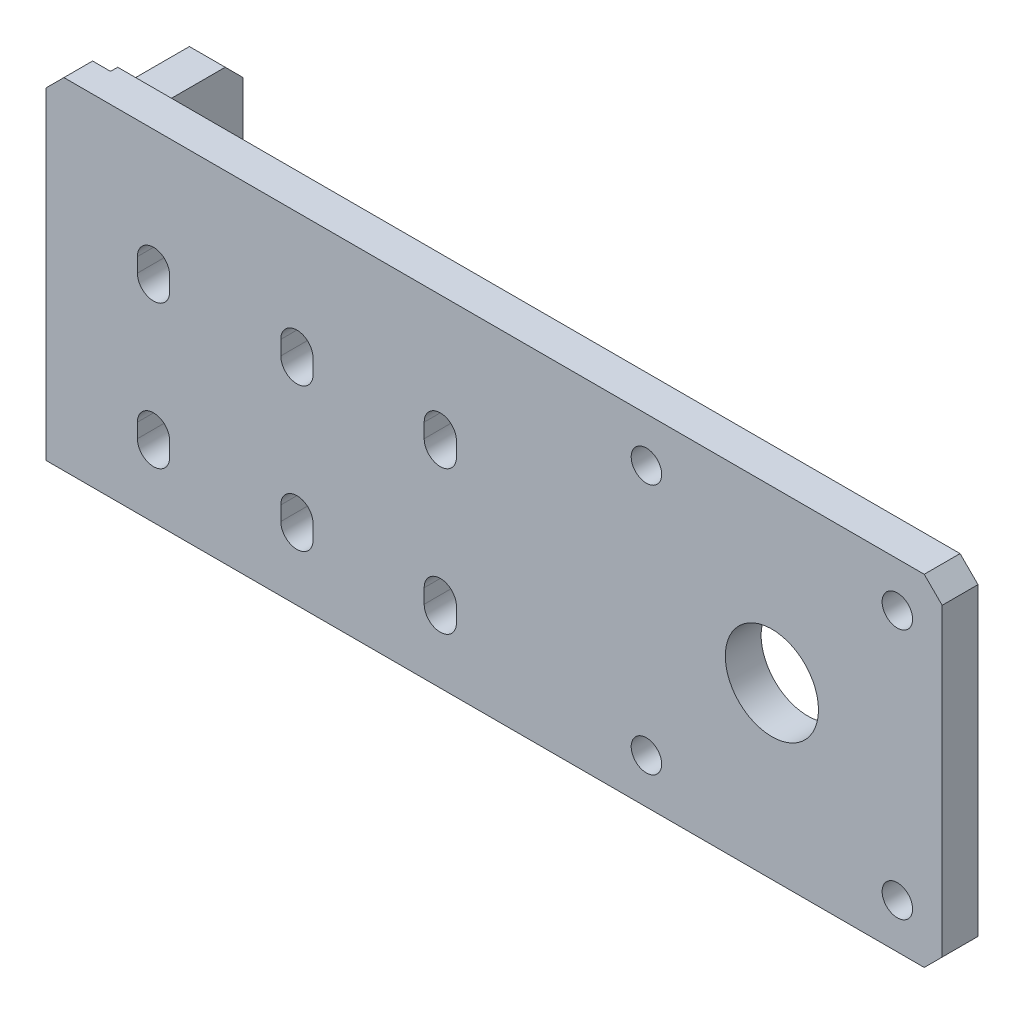
SolidWorks part; units mm, degrees
material "AISI 1045 钢，冷拔"
ref_plane "前视基准面" through (0, 0, 0) normal (0, 0, 1) x (1, 0, 0)
ref_plane "上视基准面" through (0, 0, 0) normal (0, 1, 0) x (1, 0, 0)
ref_plane "右视基准面" through (0, 0, 0) normal (1, 0, 0) x (0, 0, -1)
sketch "草图1" plane through (0, 0, 0) normal (0, 0, 1) x (1, 0, 0)
  line L1 (-125, 47.5) -> (125, 47.5)
  line L2 (-125, 47.5) -> (-125, -47.5)
  line L3 (-125, -47.5) -> (125, -47.5)
  line L4 (125, 47.5) -> (125, -47.5)
  line L5 (-125, 47.5) -> (125, -47.5) construction
  line L6 (-125, -47.5) -> (125, 47.5) construction
  point P0 (0, 0)
  dimension "D1" = 95
  dimension "D2" = 250
extrude "凸台-拉伸1" add sketch "草图1" along normal blind 10
sketch "草图3" plane through (0, 0, 10) normal (0, 0, 1) x (1, 0, 0)
  line L0 (-55, 17.5058) -> (-55, -69.5405) construction
  line L1 (125, -47.5) -> (125, 47.5) construction
  line L2 (-22.9727, -29.5) -> (-57.0867, -29.5) construction
  line L3 (-125, -47.5) -> (125, -47.5) construction
  line L4 (-55, -29.5) -> (-55, -25.5) construction
  line L5 (-59.5, -29.5) -> (-59.5, -25.5)
  line L6 (-50.5, -29.5) -> (-50.5, -25.5)
  arc A0 (-59.5, -29.5) -> (-50.5, -29.5) centre (-55, -29.5) ccw
  arc A1 (-50.5, -25.5) -> (-59.5, -25.5) centre (-55, -25.5) ccw
  point P10 (-55, -27.5)
  dimension "D4" = 4.5
  dimension "D1" = 180
  dimension "D2" = 18
  dimension "D3" = 4
extrude "切除-拉伸2" cut sketch "草图3" against normal through all
pattern_linear "阵列(线性)1" count 2 spacing 40 along (1, 0, 0) count 2 spacing 40 along (0, 1, 0) of "切除-拉伸2"
pattern_linear "阵列(线性)2" count 2 spacing 40 along (-1, 0, 0) count 2 spacing 40 along (0, 1, 0) of "切除-拉伸2"
sketch "草图10" plane through (0, 0, 10) normal (0, 0, 1) x (1, 0, 0)
  line L0 (24.75, 0) -> (-24.75, 0) construction
  line L1 (42.5, 35) -> (112.5, 35) construction
  line L2 (42.5, 35) -> (42.5, -35) construction
  line L3 (42.5, -35) -> (112.5, -35) construction
  line L4 (112.5, 35) -> (112.5, -35) construction
  line L5 (42.5, 35) -> (112.5, -35) construction
  line L6 (42.5, -35) -> (112.5, 35) construction
  line L7 (125, -47.5) -> (125, 47.5) construction
  point P0 (77.5, 0)
  dimension "D1" = 70
  dimension "D2" = 70
  dimension "D3" = 47.5
hole_wizard "M10 螺纹孔3" positions "3D草图3" profile "草图11" tap size "M10" standard "GB"
sketch3d "3D草图3"
  point P0 (42.5, 35, 10)
  point P3 (112.5, 35, 10)
  point P6 (112.5, -35, 10)
  point P9 (42.5, -35, 10)
sketch "草图11" plane through (42.5, 35, 10) normal (1, 0, 0) x (0, -1, 0)
  line L0 (0, 0) -> (0, 27.0537)
  line L1 (0, 27.0537) -> (4.25, 24.5)
  line L2 (4.25, 24.5) -> (4.25, 0)
  line L5 (4.25, 0) -> (0, 0)
  line L10 (0, 27.0537) -> (-4.25, 24.5) construction
  line L11 (0, -6.35) -> (0, 107.95) construction
  dimension "螺纹孔钻头直径" = 8.5
  dimension "螺纹孔钻头深度" = 24.5
  dimension "导头角度" = 118
cosmetic thread "孔螺蚊线9"
cosmetic thread "孔螺蚊线10"
cosmetic thread "孔螺蚊线11"
cosmetic thread "孔螺蚊线12"
sketch "草图12" plane through (0, 0, 10) normal (0, 0, 1) x (1, 0, 0)
  line L0 (42.5, 35) -> (112.5, -35) construction
  circle A0 centre (77.5, 0) radius 13
  dimension "D1" = 26
extrude "切除-拉伸5" cut sketch "草图12" against normal through all
sketch "草图13" plane through (0, 0, 0) normal (0, 0, -1) x (-1, 0, 0)
  line L0 (-45, -20) -> (-110, -20) construction
  line L1 (-110, -20) -> (-110, 20) construction
  line L2 (-110, 20) -> (-45, 20) construction
hole_wizard "M6 螺纹孔1" positions "3D草图4" profile "草图14" tap size "M6" standard "GB"
sketch3d "3D草图4"
  point P0 (45, -20, 0)
  point P3 (110, -20, 0)
  point P6 (110, 20, 0)
  point P9 (45, 20, 0)
sketch "草图14" plane through (45, -20, 0) normal (1, 0, 0) x (0, 1, 0)
  line L0 (0, 0) -> (0, 10)
  line L1 (0, 10) -> (2.5, 10)
  line L2 (2.5, 10) -> (2.5, 0)
  line L5 (2.5, 0) -> (0, 0)
  line L11 (0, -6.35) -> (0, 107.95) construction
  dimension "通孔螺纹孔钻头直径" = 5
  dimension "通孔螺纹孔钻头深度" = 10
cosmetic thread "孔螺蚊线17" [suppressed]
cosmetic thread "孔螺蚊线18" [suppressed]
cosmetic thread "孔螺蚊线19" [suppressed]
cosmetic thread "孔螺蚊线20" [suppressed]
sketch "草图15" plane through (-125, 0, 0) normal (-1, 0, 0) x (0, 0, 1)
  line L0 (5, -37.5) -> (5, -17.5) construction
  line L1 (5, -17.5) -> (5, 2.5) construction
  line L2 (5, 2.5) -> (5, 22.5) construction
hole_wizard "M6 螺纹孔2" positions "3D草图5" profile "草图16" tap size "M6" standard "GB"
sketch3d "3D草图5"
  point P0 (-125, -37.5, 5)
  point P3 (-125, -17.5, 5)
  point P6 (-125, 2.5, 5)
  point P9 (-125, 22.5, 5)
sketch "草图16" plane through (-125, -37.5, 5) normal (0, 1, 0) x (0, 0, 1)
  line L0 (0, 0) -> (0, 16.5022)
  line L1 (0, 16.5022) -> (2.5, 15)
  line L2 (2.5, 15) -> (2.5, 0)
  line L5 (2.5, 0) -> (0, 0)
  line L10 (0, 16.5022) -> (-2.5, 15) construction
  line L11 (0, -6.35) -> (0, 107.95) construction
  dimension "螺纹孔钻头直径" = 5
  dimension "螺纹孔钻头深度" = 15
  dimension "导头角度" = 118
cosmetic thread "孔螺蚊线21" [suppressed]
cosmetic thread "孔螺蚊线22" [suppressed]
cosmetic thread "孔螺蚊线23" [suppressed]
cosmetic thread "孔螺蚊线24" [suppressed]
sketch "草图18" plane through (0, -47.5, 0) normal (0, -1, 0) x (1, 0, 0)
  line L0 (12, 5) -> (47, 5) construction
  line L1 (47, 5) -> (82, 5) construction
  line L2 (82, 5) -> (117, 5) construction
  point P4 (64.5, 5)
hole_wizard "M4 螺纹孔1" positions "3D草图6" profile "草图19" tap size "M4" standard "GB"
sketch3d "3D草图6"
  point P0 (117, -47.5, 5)
  point P9 (12, -47.5, 5)
  point P12 (64.5, -47.5, 5)
sketch "草图19" plane through (117, -47.5, 5) normal (1, 0, 0) x (0, 0, -1)
  line L0 (0, 0) -> (0, 11.0914)
  line L1 (0, 11.0914) -> (1.65, 10.1)
  line L2 (1.65, 10.1) -> (1.65, 0)
  line L5 (1.65, 0) -> (0, 0)
  line L10 (0, 11.0914) -> (-1.65, 10.1) construction
  line L11 (0, -6.35) -> (0, 107.95) construction
  dimension "螺纹孔钻头直径" = 3.3
  dimension "螺纹孔钻头深度" = 10.1
  dimension "导头角度" = 118
cosmetic thread "孔螺蚊线25"
cosmetic thread "孔螺蚊线26"
cosmetic thread "孔螺蚊线28"
sketch "草图22" plane through (0, 0, 0) normal (0, 0, -1) x (-1, 0, 0)
  line L0 (125, -47.5) -> (-125, -47.5) construction
  line L1 (125, 47.5) -> (115, 47.5)
  line L2 (125, 47.5) -> (125, -47.5)
  line L3 (125, -47.5) -> (115, -47.5)
  line L4 (115, 47.5) -> (115, -47.5)
  dimension "D1" = 10
extrude "切除-拉伸6" cut sketch "草图22" against normal blind 2
sketch "草图21" plane through (0, 0, 2) normal (0, 0, -1) x (-1, 0, 0)
  line L1 (125, -47.5) -> (115, -47.5)
  line L2 (125, -47.5) -> (125, 32.5)
  line L3 (125, 32.5) -> (115, 32.5)
  line L4 (115, -47.5) -> (115, 32.5)
  dimension "D1" = 80
  dimension "D2" = 10
extrude "凸台-拉伸2" add sketch "草图21" along normal blind 37 separate body
chamfer "倒角1" distance 5 angle 45 3 edges at (125, -47.5, 5) (125, 47.5, 5) (-125, 47.5, 6)
chamfer "倒角2" distance 5 angle 45 2 edges at (-120, 32.5, -35) (-120, -47.5, -35)
